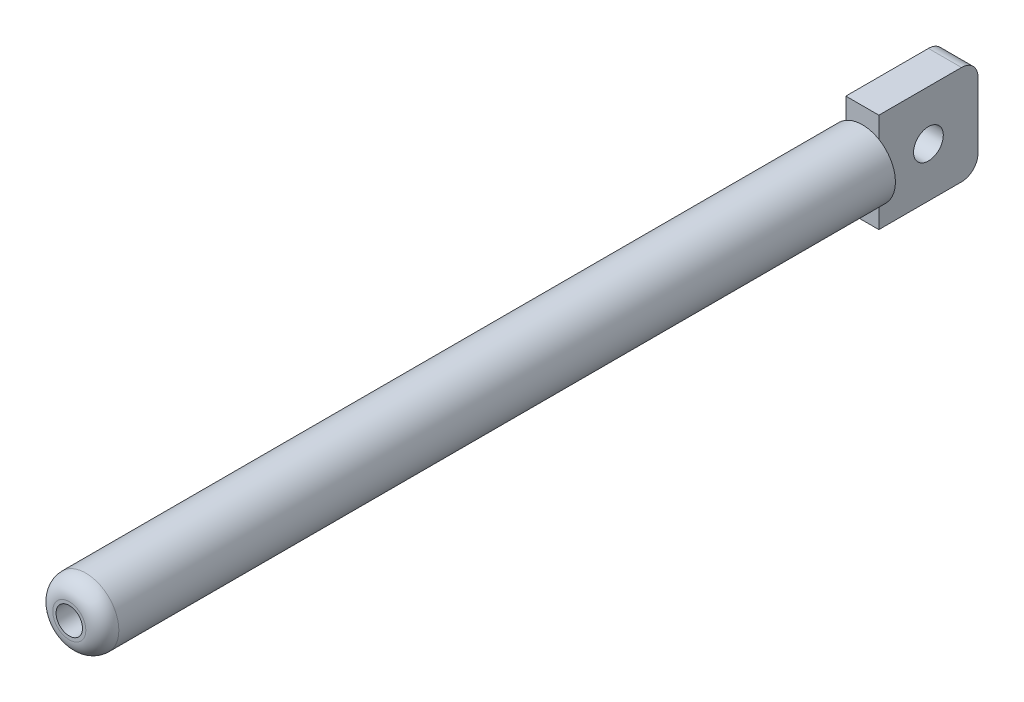
from build123d import *

# Parameters (mm, degrees)
SKETCH1_R           = 10
BOSS_EXTRUDE1_DEPTH = 240
SKETCH2_W           = 30
SKETCH2_H           = 30
BOSS_EXTRUDE2_DEPTH = 5
SKETCH3_R           = 4.5
CUT_EXTRUDE1_DEPTH  = 38
FILLET1_R           = 5
FILLET2_R           = 5
SKETCH4_R           = 4
CUT_EXTRUDE2_DEPTH  = 20


with BuildPart() as part:
    # Sketch1 → Boss-Extrude1 (new body)
    with BuildSketch(Plane.XY):
        Circle(SKETCH1_R)
    extrude(amount=BOSS_EXTRUDE1_DEPTH)

    # Sketch2 → Boss-Extrude2 (add, symmetric)
    with BuildSketch(Plane(origin=(0, 0, 0), x_dir=(0, 0, -1), z_dir=(1, 0, 0))):
        with Locations((15, 0)):
            Rectangle(SKETCH2_W, SKETCH2_H)
    extrude(amount=BOSS_EXTRUDE2_DEPTH, both=True)

    # Sketch3 → Cut-Extrude1 (cut)
    with BuildSketch(Plane(origin=(5, 0, 0), x_dir=(0, 0, -1), z_dir=(1, 0, 0))):
        with Locations((15, 0)):
            Circle(SKETCH3_R)
    extrude(amount=-CUT_EXTRUDE1_DEPTH, mode=Mode.SUBTRACT)

    # Fillet1
    fillet1_edges = [part.edges().sort_by_distance(p)[0] for p in [
        (0, -15, -30),
        (0, 15, -30),
    ]]
    fillet(fillet1_edges, radius=FILLET1_R)

    # Fillet2
    fillet2_edges = [part.edges().sort_by_distance(p)[0] for p in [
        (-10, 0, 240),
    ]]
    fillet(fillet2_edges, radius=FILLET2_R)

    # Sketch4 → Cut-Extrude2 (cut)
    with BuildSketch(Plane.XY.offset(240)):
        Circle(SKETCH4_R)
    extrude(amount=-CUT_EXTRUDE2_DEPTH, mode=Mode.SUBTRACT)


solid = part.part
